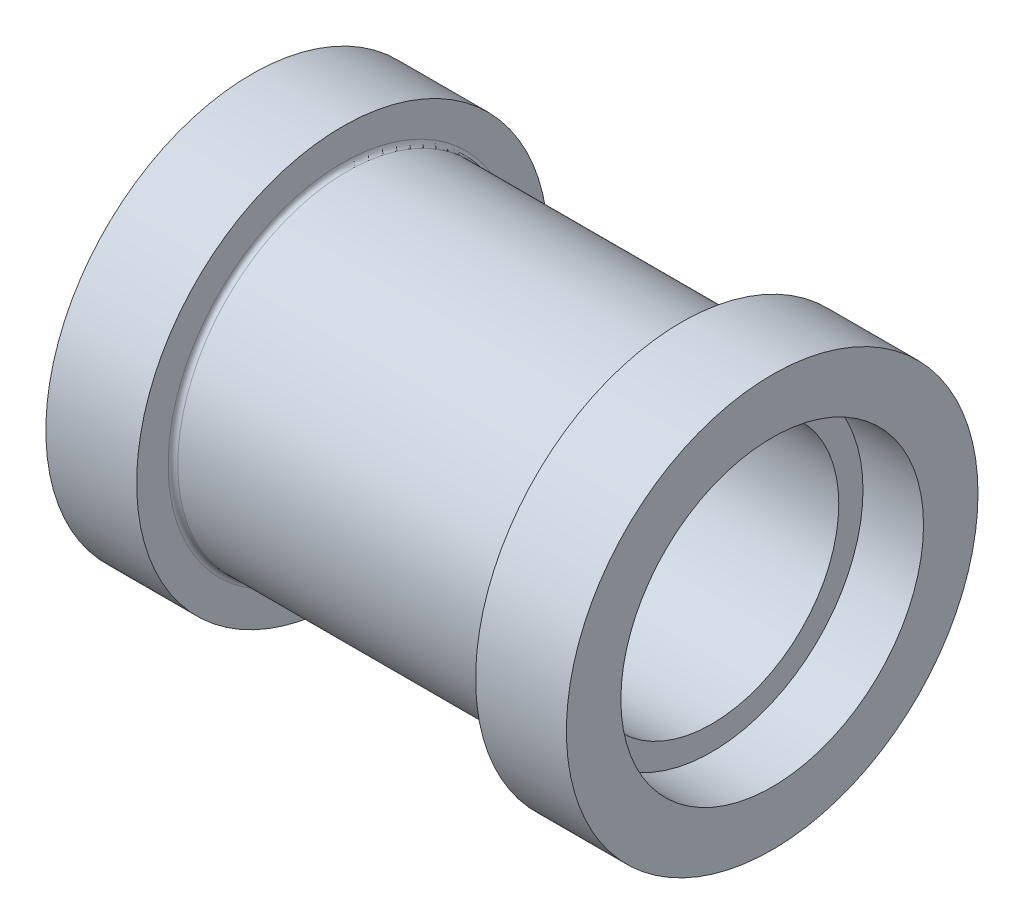
SolidWorks part; units mm, degrees
material "普通碳钢"
ref_plane "Front Plane" through (0, 0, 0) normal (0, 0, 1) x (1, 0, 0)
ref_plane "Top Plane" through (0, 0, 0) normal (0, 1, 0) x (1, 0, 0)
ref_plane "Right Plane" through (0, 0, 0) normal (1, 0, 0) x (0, 0, -1)
other "Configuration Table"
sketch "Sketch1" plane through (0, 0, 0) normal (1, 0, 0) x (0, 0, -1)
  circle A0 centre (0, 0) radius 85
  dimension "D1" = 170
extrude "Boss-Extrude1" add sketch "Sketch1" along normal blind 215
ref_plane "Plane1" through (172.5, 0, 0) normal (1, 0, 0) x (0, 0, -1)
sketch "Sketch2" plane through (172.5, 0, 0) normal (1, 0, 0) x (0, 0, -1)
  circle A0 centre (0, 0) radius 70
  circle A1 centre (0, 0) radius 110
  dimension "D1" = 140
  dimension "D2" = 220
extrude "Cut-Extrude1" cut sketch "Sketch2" against normal blind 140 from offset 5
fillet "Fillet1" radius 2 2 edges at (177.5, 0, -70) (37.5, 0, -70)
sketch "Sketch3" plane through (215, 0, 0) normal (1, 0, 0) x (0, 0, -1)
  circle A0 centre (0, 0) radius 62.5
  dimension "D1" = 125
extrude "Cut-Extrude2" cut sketch "Sketch3" against normal blind 25
sketch "Sketch4" plane through (0, 0, 0) normal (-1, 0, 0) x (0, 0, 1)
  circle A0 centre (0, 0) radius 62.5
  dimension "D1" = 125
extrude "Cut-Extrude3" cut sketch "Sketch4" against normal blind 25
sketch "Sketch5" plane through (190, 0, 0) normal (1, 0, 0) x (0, 0, -1)
  circle A0 centre (0, 0) radius 52.5
  dimension "D1" = 105
extrude "Cut-Extrude4" cut sketch "Sketch5" against normal through all
